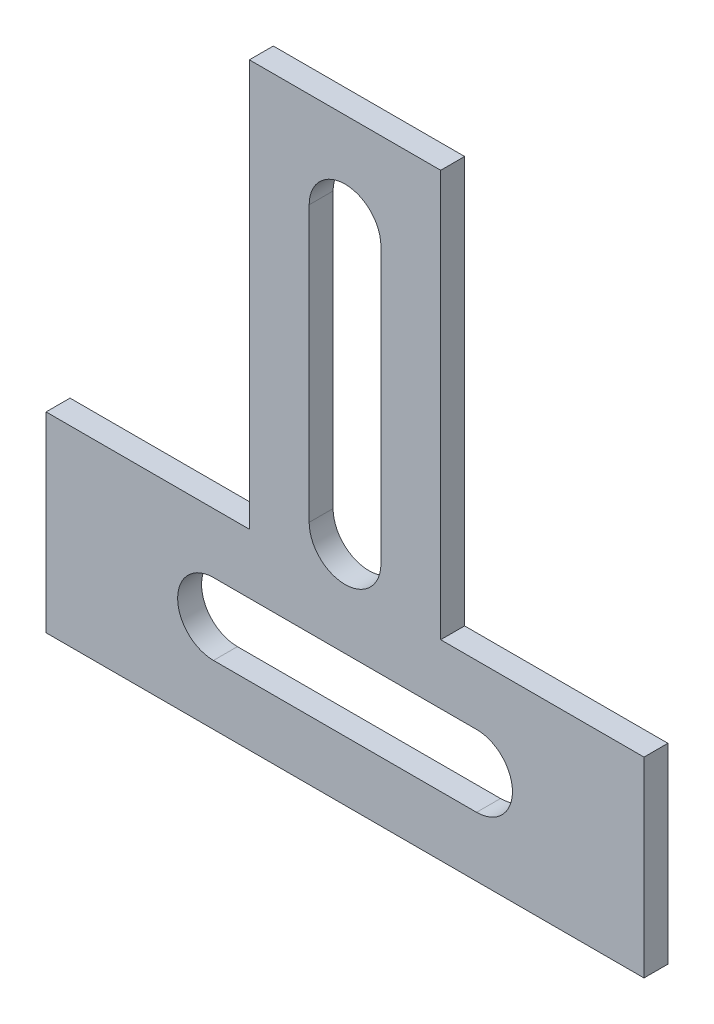
SolidWorks part; units mm, degrees
ref_plane "前视基准面" through (0, 0, 0) normal (0, 0, 1) x (1, 0, 0)
ref_plane "上视基准面" through (0, 0, 0) normal (0, 1, 0) x (1, 0, 0)
ref_plane "右视基准面" through (0, 0, 0) normal (1, 0, 0) x (0, 0, -1)
sketch "草图1" plane through (0, 0, 0) normal (0, 0, 1) x (1, 0, 0)
  line L0 (0, 20) -> (0, 0) construction
  line L1 (25, -8) -> (-25, -8)
  line L2 (25, -8) -> (25, 8)
  line L3 (25, 8) -> (8, 8)
  line L4 (-25, -8) -> (-25, 8)
  line L5 (25, -8) -> (-25, 8) construction
  line L6 (25, 8) -> (-25, -8) construction
  line L7 (8, 42) -> (-8, 42)
  line L8 (8, 42) -> (8, 8)
  line L10 (-8, 42) -> (-8, 8)
  line L11 (8, 42) -> (-8, 8) construction
  line L12 (8, 8) -> (-8, 42) construction
  line L13 (0, 11) -> (0, 34) construction
  line L14 (-3, 11) -> (-3, 34)
  line L15 (3, 11) -> (3, 34)
  line L16 (-11, 0) -> (11, 0) construction
  line L17 (-11, 3) -> (11, 3)
  line L18 (-11, -3) -> (11, -3)
  line L19 (-8, 8) -> (-25, 8)
  arc A0 (-3, 11) -> (3, 11) centre (0, 11) ccw
  arc A1 (3, 34) -> (-3, 34) centre (0, 34) ccw
  arc A2 (-11, 3) -> (-11, -3) centre (-11, 0) ccw
  arc A3 (11, -3) -> (11, 3) centre (11, 0) ccw
  point P0 (0, 0)
  point P15 (0, 22.5)
  point P21 (0, 0)
  dimension "D1" = 50
  dimension "D2" = 17
  dimension "D3" = 34
  dimension "D4" = 50
  dimension "D5" = 6
  dimension "D6" = 22
  dimension "D7" = 23
extrude "凸台-拉伸2" add sketch "草图1" along normal blind 2
